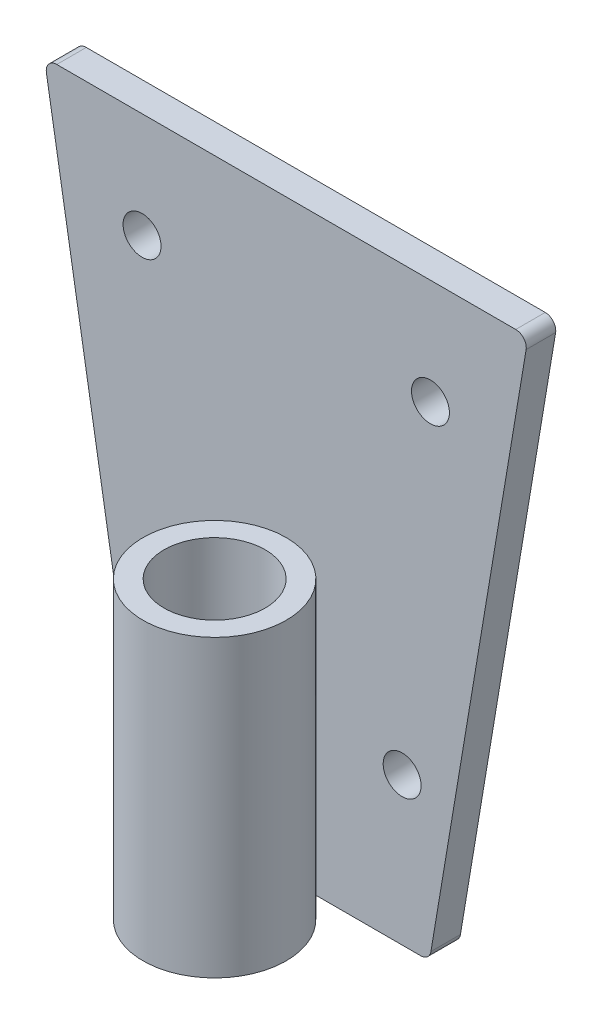
from build123d import *

# Parameters (mm, degrees)
EXTRUDE_1_DEPTH                  = 14
SKETCH_2_R                       = 34
SKETCH_2_R_2                     = 24
EXTRUDE_2_DEPTH                  = 140
FILLET_1_R                       = 5
HOLE_WIZARD_18_0_18_1_AT_2_COUNT = 2
HOLE_WIZARD_18_0_18_1_AT_2_PITCH = 160.563264727
HOLE_WIZARD_18_0_18_1_AT_3_COUNT = 2
HOLE_WIZARD_18_0_18_1_AT_3_PITCH = 202.081111798
HOLE_WIZARD_18_0_18_1_AT_4_COUNT = 2
HOLE_WIZARD_18_0_18_1_AT_4_PITCH = 136.874670595


with BuildPart() as part:
    # 草图1 → 凸台-拉伸1 (new body)
    with BuildSketch(Plane.XY):
        Polygon((-67.968990431, -2335), (67.968990431, -2335), (114.824920973, -2055), (-114.824920973, -2055), align=None)
    extrude(amount=EXTRUDE_1_DEPTH)

    # 圆角1
    fillet_1_edges = [part.edges().sort_by_distance(p)[0] for p in [
        (-114.824920973, -2055, 7),
        (114.824920973, -2055, 7),
        (67.968990431, -2335, 7),
        (-67.968990431, -2335, 7),
    ]]
    fillet(fillet_1_edges, radius=FILLET_1_R)

    # 草图5 → Ø18.0 (18) 直径孔1 (revolve, cut)
    with BuildSketch(Plane(origin=(68.437335298, -2105, 0), x_dir=(0, 1, 0), z_dir=(1, 0, 0))):
        Polygon((0, 0), (0, 65.407745571), (9, 60), (9, 0), align=None)
    hole_wizard_18_0_18_1 = revolve(axis=Axis((68.437335298, -2105, -6.35), (0, 0, 1)), mode=Mode.SUBTRACT)

    # Ø18.0 (18) 直径孔1 at 2: Ø18.0 (18) 直径孔1 ×2
    with Locations(*[Vector(-0.08368872743367663, -0.9964919452261176, 0) * (i * HOLE_WIZARD_18_0_18_1_AT_2_PITCH) for i in range(1, HOLE_WIZARD_18_0_18_1_AT_2_COUNT)]):
        add(hole_wizard_18_0_18_1, mode=Mode.SUBTRACT)

    # Ø18.0 (18) 直径孔1 at 3: Ø18.0 (18) 直径孔1 ×2
    with Locations(*[Vector(-0.6108306422087694, -0.7917612812829524, 0) * (i * HOLE_WIZARD_18_0_18_1_AT_3_PITCH) for i in range(1, HOLE_WIZARD_18_0_18_1_AT_3_COUNT)]):
        add(hole_wizard_18_0_18_1, mode=Mode.SUBTRACT)

    # Ø18.0 (18) 直径孔1 at 4: Ø18.0 (18) 直径孔1 ×2
    with Locations(*[(-i * HOLE_WIZARD_18_0_18_1_AT_4_PITCH, 0, 0) for i in range(1, HOLE_WIZARD_18_0_18_1_AT_4_COUNT)]):
        add(hole_wizard_18_0_18_1, mode=Mode.SUBTRACT)


with BuildPart() as body_2:
    # 草图2 → 凸台-拉伸2 (new body)
    with BuildSketch(Plane.XZ.offset(2335)):
        with Locations(Location((0, 48, 0), (0, 0, 270))):
            Circle(SKETCH_2_R)
        with Locations(Location((0, 48, 0), (0, 0, 270))):
            Circle(SKETCH_2_R_2, mode=Mode.SUBTRACT)
    extrude(amount=-EXTRUDE_2_DEPTH)


solid = Compound([part.part, body_2.part])
